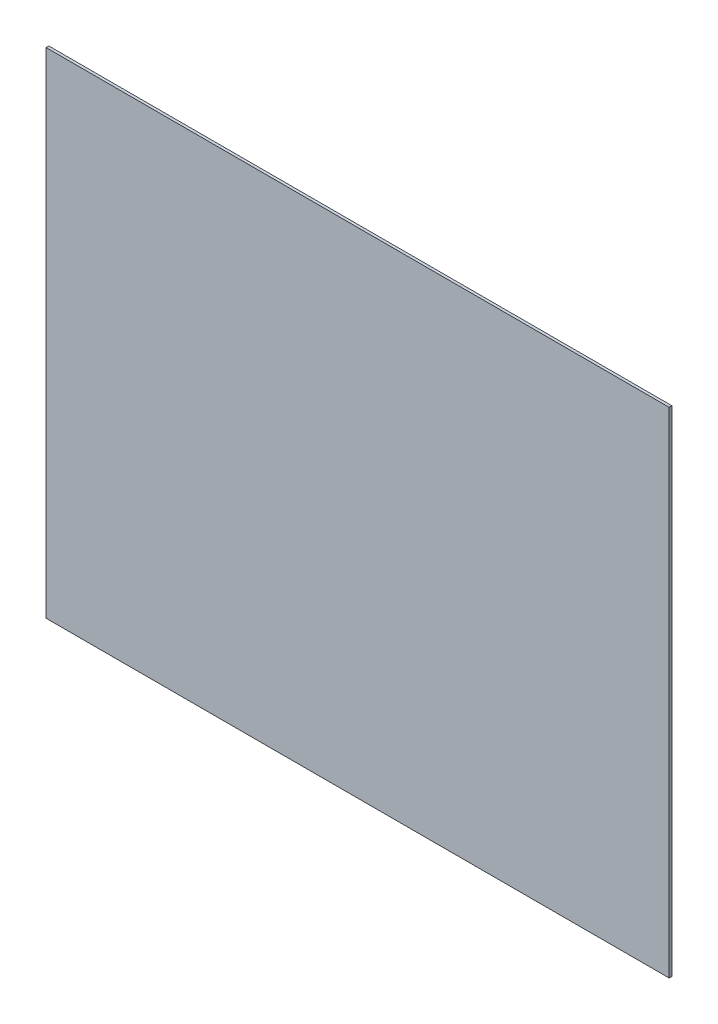
from build123d import *

# Parameters (mm, degrees)
SKETCH_1_W      = 1142
SKETCH_1_H      = 906
EXTRUDE_1_DEPTH = 5


with BuildPart() as part:
    # 草图1 → 凸台-拉伸1 (new body)
    with BuildSketch(Plane.XY):
        Rectangle(SKETCH_1_W, SKETCH_1_H)
    extrude(amount=EXTRUDE_1_DEPTH)


solid = part.part
